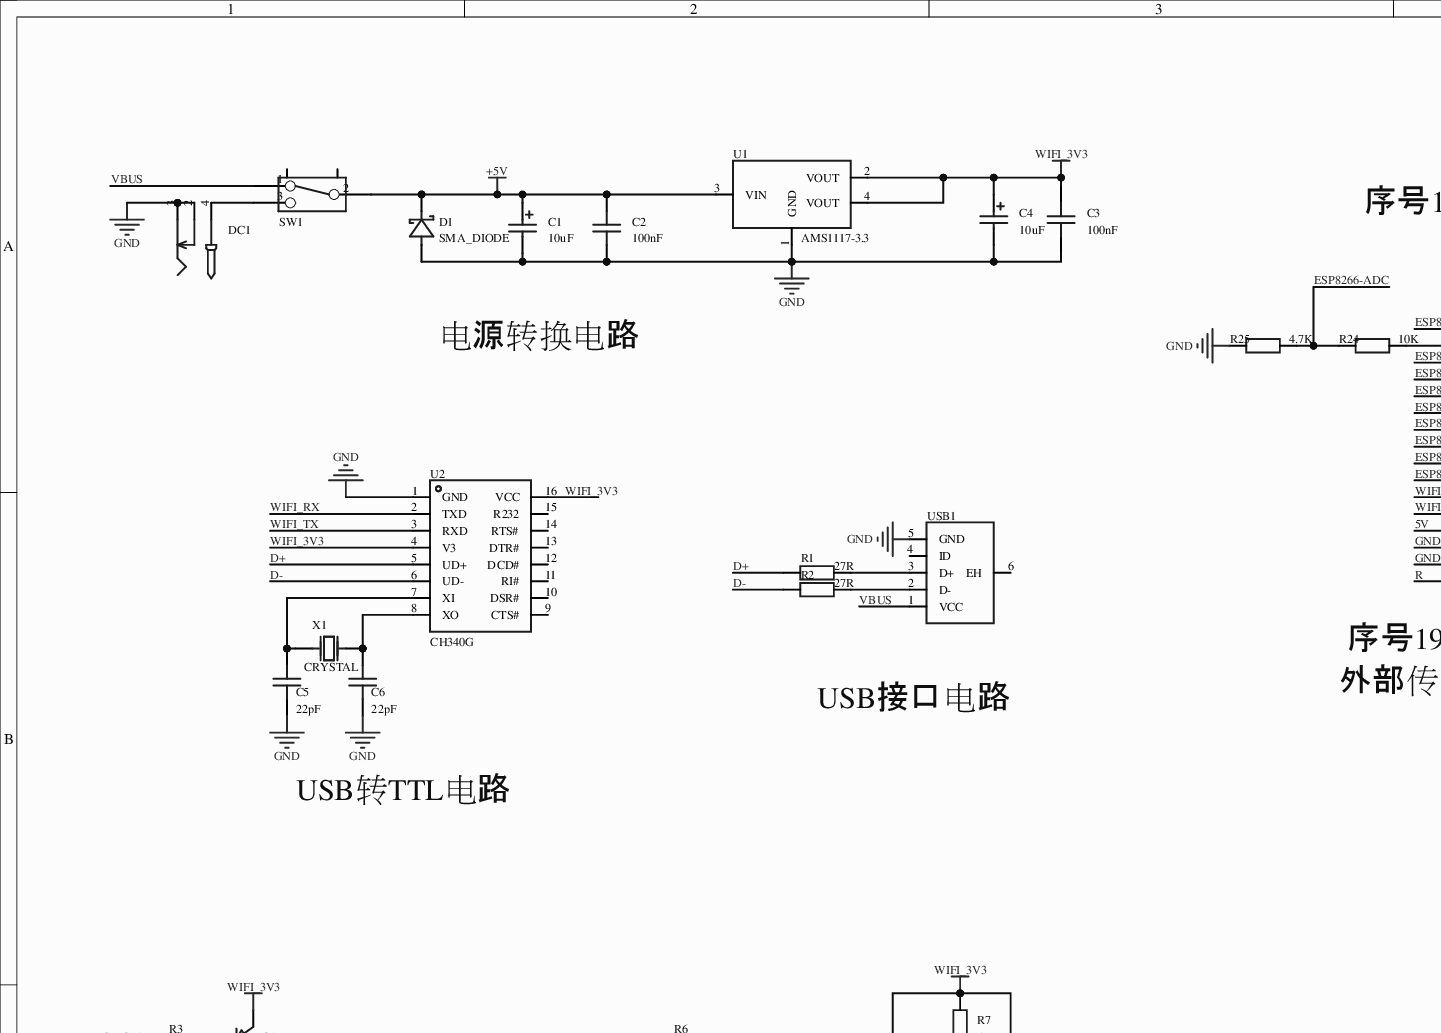
[diagram p0: MISC51905-3.schdoc, top left]
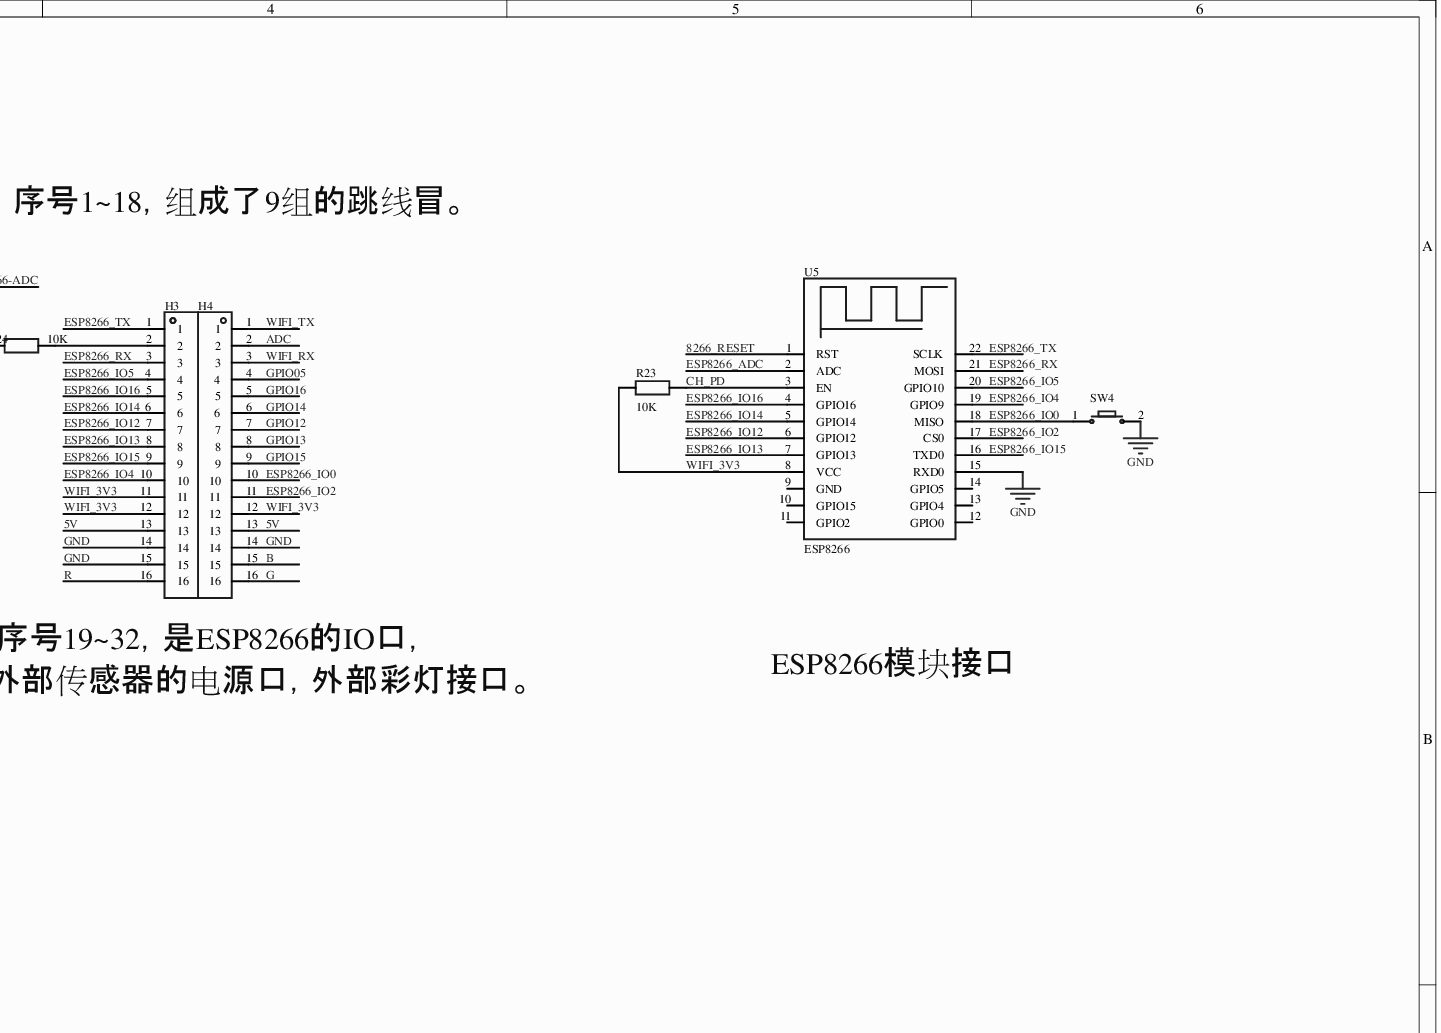
[diagram p1: MISC51905-3.schdoc, top right]
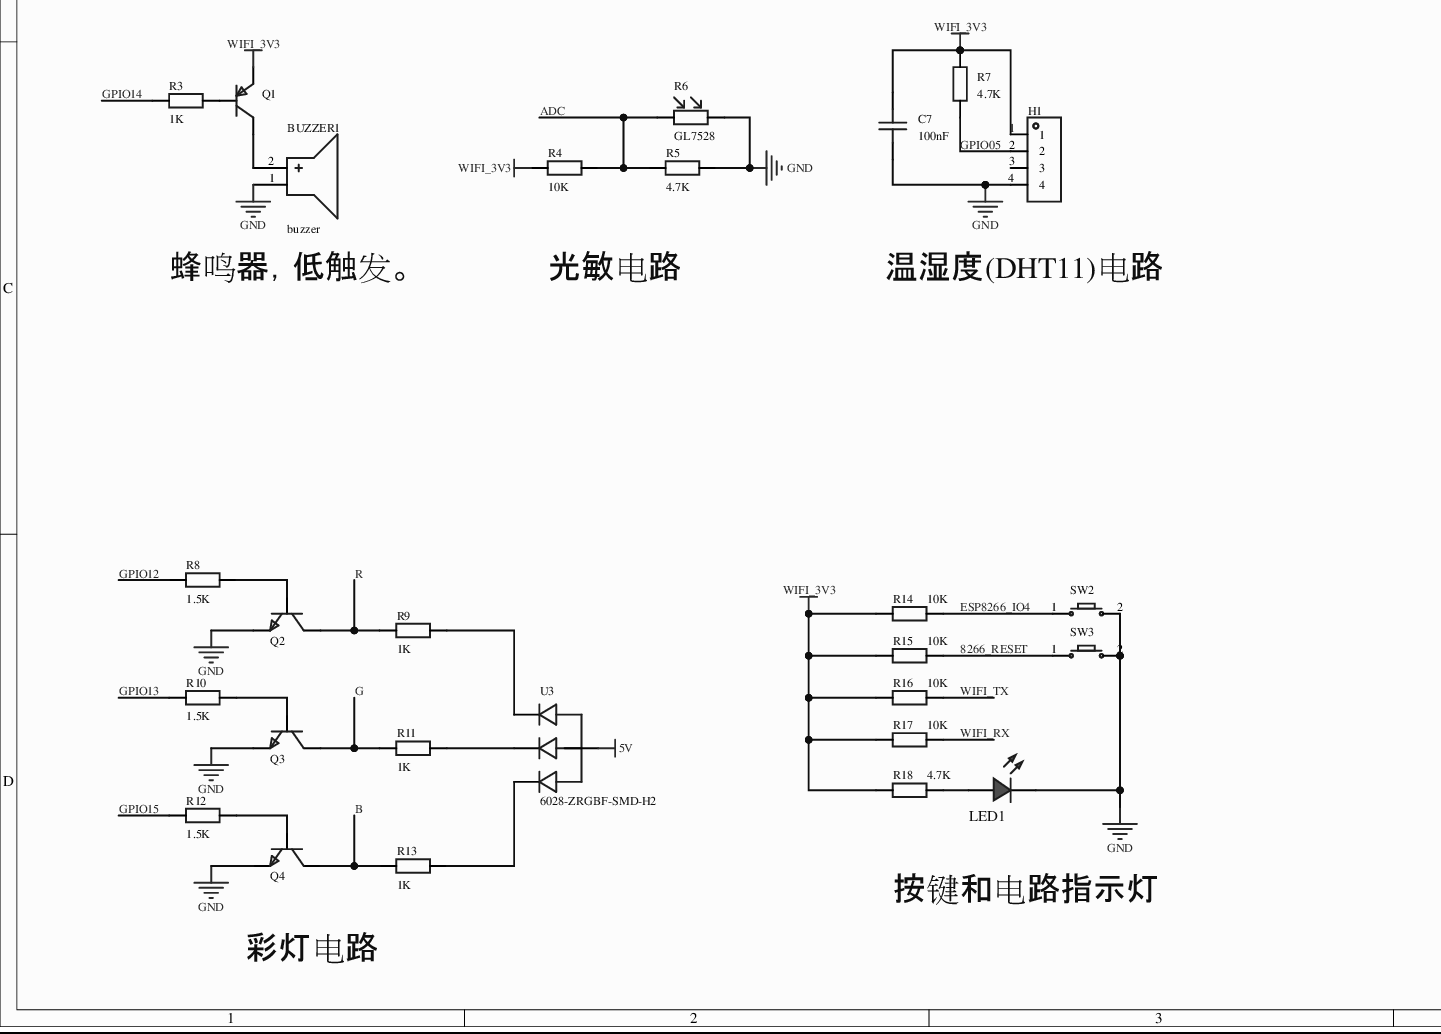
[diagram p2: MISC51905-3.schdoc, bottom left]
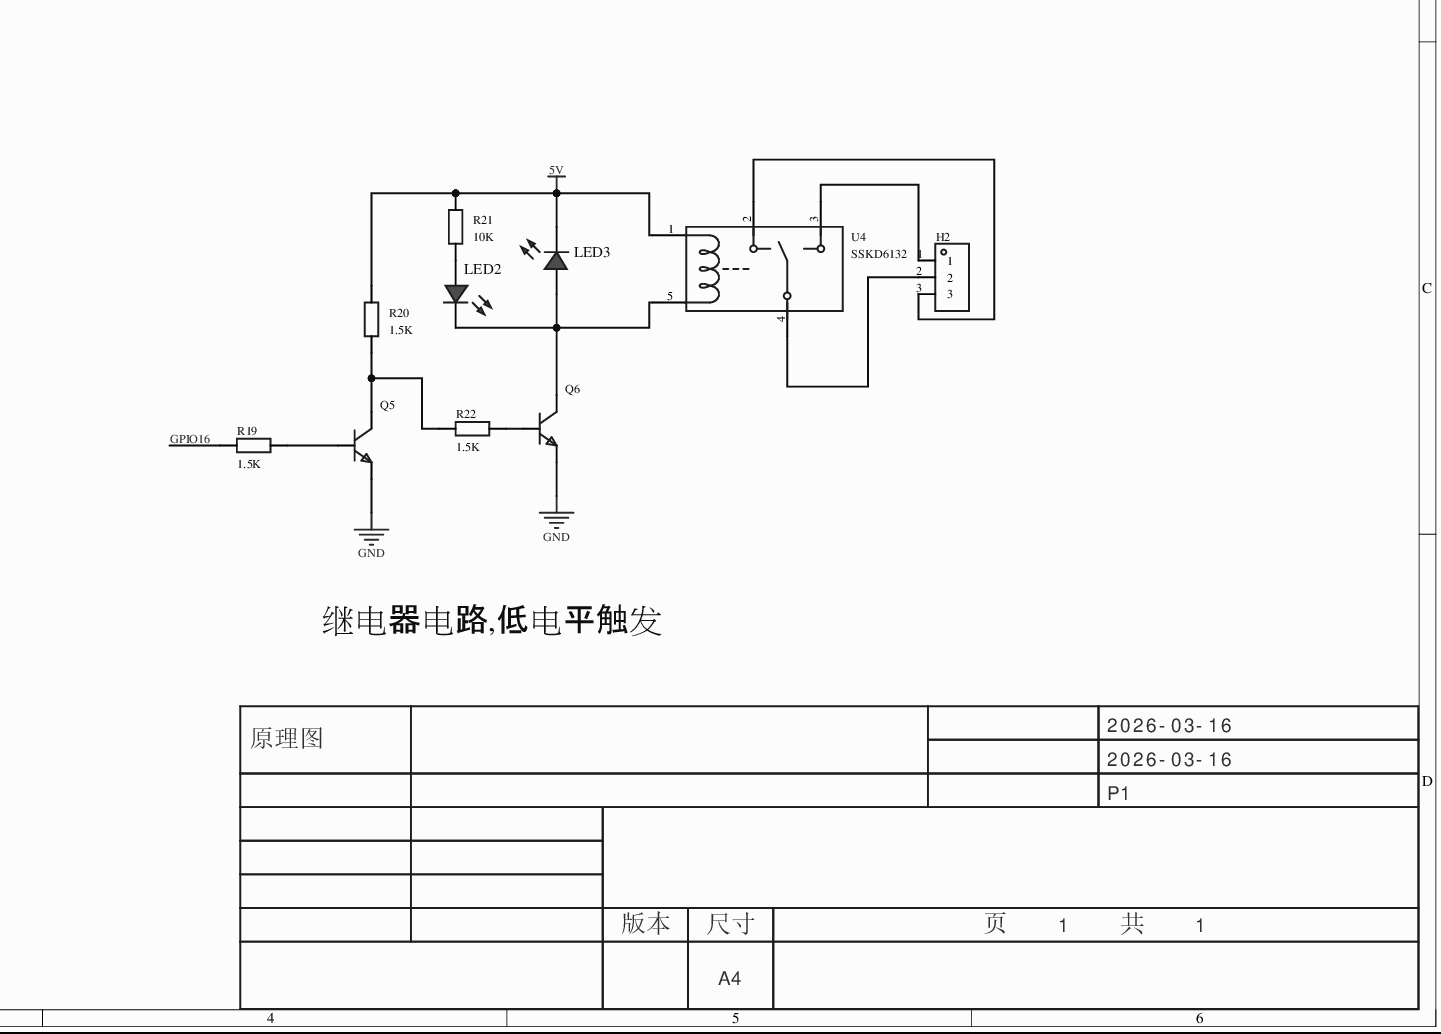
[diagram p3: MISC51905-3.schdoc, bottom right]
# Altium project MISC51905-2.PrjPcb
1 sheet, 59 parts. Net scope: global (net labels, ports and power ports of the same name join across sheets).
Board file: MISC51905.pcbdoc

## Sheet MISC51905-3.schdoc
size 420 x 297 mm; Version: V1.0; @Project Name: MISC51905; @Update Date: 2026-03-16; @Create Date: 2026-03-16; @Board Name: MISC51905; @Create Time: 19:00:49; @Page Count: 1; @Page No: 1; @Schematic Name: MISC51905; @Update Time: 19:00:49; Size: A4

### Parts
BUZZER1  buzzer  [BUZ-TH_BD12.0-P6.00-D0.9-RD]
C1  10uF  [C_Ele_SMD_5x5.4mm]
C2  100nF  [C0603]
C3  100nF  [C0603]
C4  10uF  [C_Ele_SMD_5x5.4mm]
C5  22pF  [C0603]
C6  22pF  [C0603]
C7  100nF  [C0603]
D1  SMA_DIODE  [SOD-57_BD3.8-L4.6-P9.00-D0.8-RD]
DC1  (no value)  [DC-2.0]
H1  (no value)  [HDR-TH_4P-P2.54-V-F]
H2  (no value)  [HDR-TH_3P-P2.54-V-F]
H3  (no value)  [HDR-TH_16P-P2.54-V-F]
H4  (no value)  [HDR-TH_16P-P2.54-V-F]
LED1  (no value)  [LED_0805]
LED2  (no value)  [LED_0805]
LED3  (no value)  [LED_0805]
Q1  (no value)  [S8550P_SOT]
Q2  (no value)  [S8050_SOT-23]
Q3  (no value)  [S8050_SOT-23]
Q4  (no value)  [S8050_SOT-23]
Q5  (no value)  [S8050_SOT-23]
Q6  (no value)  [S8050_SOT-23]
R1  27R  [R0603]
R2  27R  [R0603]
R3  1K  [R0805]
R4  10K  [R0805]
R5  4.7K  [R0805]
R6  GL7528  [RES-TH_L7.0-W5.9-P5.00-D0.5]
R7  4.7K  [R0805]
R8  1.5K  [R0805]
R9  1K  [R0805]
R10  1.5K  [R0805]
R11  1K  [R0805]
R12  1.5K  [R0805]
R13  1K  [R0805]
R14  10K  [R0805]
R15  10K  [R0805]
R16  10K  [R0805]
R17  10K  [R0805]
R18  4.7K  [R0805]
R19  1.5K  [R0805]
R20  1.5K  [R0805]
R21  10K  [R0805]
R22  1.5K  [R0805]
R23  10K  [R0805]
R24  10K  [Res_1/8W]
R25  4.7K  [Res_1/8W]
SW1  (no value)  [拨动开关_侧]
SW2  (no value)  [Key_SMD_3x4x2]
SW3  (no value)  [Key_SMD_3x4x2]
SW4  (no value)  [Key_SMD_3x4x2]
U1  AMS1117-3.3  [SOT-223-3_L6.5-W3.4-P2.30-LS7.0-BR]
U2  CH340G  [SOIC-16_L9.9-W3.9-P1.27-LS6.0-BL]
U3  6028-ZRGBF-SMD-H2  [LED-SMD_4P-L3.2-W2.8_ZRGBF-SMD-H2]
U4  SSKD6132  [RELAY-TH_G2R-1]
U5  ESP8266  [WIFIM-SMD_ESP-12F-ESP8266MOD]
USB1  (no value)  [USB_Micro]
X1  CRYSTAL  [CRYSTAL-SMD_L5.0-W3.2]

### Nets
5V: H3.13 H4.13 LED3.1(C) R20.2 R21.2 U3.2(COM+) U4.1
+5V: C1.1 C2.2 D1.1(K) SW1.2 U1.3(VIN)
GND: BUZZER1.1(-) C1.2 C2.1 C3.1 C4.2 C5.1 C6.1 C7.1 D1.2(A) DC1.2 DC1.3 H1.4 H3.14 H3.15 H4.14 LED1.1(C) Q2.2 Q3.2 Q4.2 Q5.2 Q6.2 R5.2 R6.2 R25.1 SW2.2 SW3.2 SW4.2 U1.1(GND) U2.1(GND) U5.15(RXD0) USB1.5(GND)
WIFI_3V3: C3.2 C4.1 C7.2 H1.1 H3.11 H3.12 H4.12 Q1.2(E) R4.1 R7.2 R14.1 R15.1 R16.1 R17.1 R18.1 R23.1 U1.2(VOUT) U1.4(VOUT) U2.4(V3) U2.16(VCC) U5.8(VCC)
8266_RESET: R15.2 SW3.1 U5.1(RST)
ADC: H4.2 R4.2 R5.1 R6.1
B: H4.15 Q4.3 R13.1
CH_PD: R23.2 U5.3(EN)
D+: R1.1 U2.5(UD+)
D-: R2.1 U2.6(UD-)
ESP8266-ADC: R24.1 R25.2
ESP8266_ADC: U5.2(ADC)
ESP8266_IO0: H4.10 SW4.1 U5.18(MISO)
ESP8266_IO2: H4.11 U5.17(CS0)
ESP8266_IO4: H3.10 R14.2 SW2.1 U5.19(GPIO9)
ESP8266_IO5: H3.4 U5.20(GPIO10)
ESP8266_IO12: H3.7 U5.6(GPIO12)
ESP8266_IO13: H3.8 U5.7(GPIO13)
ESP8266_IO14: H3.6 U5.5(GPIO14)
ESP8266_IO15: H3.9 U5.16(TXD0)
ESP8266_IO16: H3.5 U5.4(GPIO16)
ESP8266_RX: H3.3 U5.21(MOSI)
ESP8266_TX: H3.1 U5.22(SCLK)
G: H4.16 Q3.3 R11.1
GPIO05: H1.2 H4.4 R7.1
GPIO12: H4.7 R8.1
GPIO13: H4.8 R10.1
GPIO14: H4.6 R3.1
GPIO15: H4.9 R12.1
GPIO16: H4.5 R19.1
R: H3.16 Q2.3 R9.1
VBUS: SW1.1 USB1.1(VCC)
WIFI_RX: H4.3 R17.2 U2.2(TXD)
WIFI_TX: H4.1 R16.2 U2.3(RXD)
NetBUZZER1_2: BUZZER1.2(+) Q1.3(C)
NetC5_2: C5.2 U2.7(XI) X1.1(OSC1)
NetC6_2: C6.2 U2.8(XO) X1.2(OSC2)
NetDC1_4: DC1.4 SW1.3
NetH2_1: H2.1 U4.3
NetH2_2: H2.2 U4.4
NetH2_3: H2.3 U4.2
NetH3_2: H3.2 R24.2
NetLED1_2: LED1.2(A) R18.2
NetLED2_1: LED2.1(C) LED3.2(A) Q6.3 U4.5
NetLED2_2: LED2.2(A) R21.1
NetQ1_1: Q1.1(B) R3.2
NetQ2_1: Q2.1 R8.2
NetQ3_1: Q3.1 R10.2
NetQ4_1: Q4.1 R12.2
NetQ5_1: Q5.1 R19.2
NetQ5_3: Q5.3 R20.1 R22.1
NetQ6_1: Q6.1 R22.2
NetR1_2: R1.2 USB1.3(D+)
NetR2_2: R2.2 USB1.2(D-)
NetR9_2: R9.2 U3.1(R)
NetR11_2: R11.2 U3.4(B)
NetR13_2: R13.2 U3.3(G)

Not connected (* = marked no-connect by the designer): H1 3; SW1 4 5; U2 9(CTS#) 10(DSR#) 11(RI#) 12(DCD#) 13(DTR#) 14(RTS#) 15(R232); U5 9(GND) 10(GPIO15) 11(GPIO2) 12(GPIO0) 13(GPIO4) 14(GPIO5); USB1 4(ID) 6(EH)

### Notes on the sheet
- 序号1~18，组成了9组的跳线冒。
- 电源转换电路
- 序号19~32，是ESP8266的IO口，
- USB接口电路
- 外部传感器的电源口，外部彩灯接口。
- ESP8266模块接口
- USB转TTL电路
- 蜂鸣器，低触发。
- 光敏电路
- 温湿度(DHT11)电路
- 继电器电路,低电平触发
- 彩灯电路
- 按键和电路指示灯
- 2026-03-16
- 原理图
- P1
- 版本
- 尺寸
- A4
- 页    1    共    1

### Library data of the parts
BUZZER1 = buzzer: AddInBom: yes; ModelId: af17e4151ed84fc2a628230bf23763630819f05c4eef4c71ace90d822a990e87; ModelTransform: 472.44,472.176,0,270,0,0,0,0,-196.85; Symbol: BUZZER; Device: buzzer; LCSC Part Name: buzzer; SupplierPart: C9900014030; ManufacturerPart: buzzer; Supplier Footprint: buzzer; JLCPCB Part Class: Extended Part; Supplier: LCSC; ConvertToPcb: yes; FootprintName: BUZ-TH_BD12.0-P6.00-D0.9-RD; ModelName: BUZ-TH_BD12.0-P6.00-D0.9-RD
C1 C4 = C_Ele_SMD_5x5.4mm: Symbol: CAP; AddInBom: yes; Device: C_Ele_SMD_5x5.4mm; Supplier Footprint: SMD,5x5.4mm; ConvertToPcb: yes; FootprintName: C_Ele_SMD_5x5.4mm; Value: 10uF
C2 C3 C5-C7 = CAP_0603: Symbol: Capacitance; ConvertToPcb: yes; ModelId: ac125912035d415993ca9572d50418b10819f05c4eef4c71ace90d822a990e87; ModelName: C0603_L1.6-W0.8-H0.8; ModelTransform: 62.992,31.496,0,0,0,0,0,0,0; Device: CAP_0603; AddInBom: yes; Supplier Footprint: 0603; FootprintName: C0603
  C2 C3 C7: Value: 100nF
  C5 C6: Value: 22pF
D1 = SMA_DIODE: AddInBom: yes; ModelId: 9d3120876592498385ffc7c85c6b53e30819f05c4eef4c71ace90d822a990e87; ModelTransform: 354.33,149.70372,0,0,0,0,0,0,-137.795; Symbol: SMA_DIODE; Device: SMA_DIODE; LCSC Part Name: SMA_DIODE; SupplierPart: C9900013997; ManufacturerPart: SMA_DIODE; Supplier Footprint: 1N4007_SMADIODE; JLCPCB Part Class: Extended Part; Supplier: LCSC; ConvertToPcb: yes; FootprintName: SOD-57_BD3.8-L4.6-P9.00-D0.8-RD; ModelName: SOD-57_BD3.8-L4.6-P9.00-D0.8-RD
DC1 = DC-005_2.0: Symbol: DC电源接口; ConvertToPcb: yes; ModelId: f5f20b8a2308479b936ba3c2698865bb0819f05c4eef4c71ace90d822a990e87; ModelName: DC-IN-TH_DC-5520-1; ModelTransform: 372.05,551.18,582.68,90,0,0,137.8,0,-149.61; Device: DC-005_2.0; AddInBom: yes; Supplier Footprint: 插件; FootprintName: DC-2.0
H1 = HDR-F_2.54_1x4P: Symbol: 2.54-1*4P母; ConvertToPcb: yes; ModelId: d187812051054f85879fcaa51a310d8e0819f05c4eef4c71ace90d822a990e87; ModelTransform: 419.6842,98.464,0,0,0,0,0,0,-118.11; Device: HDR-F_2.54_1x4P; AddInBom: yes; SupplierPart: C2718488; Supplier Footprint: 插件; FootprintName: HDR-TH_4P-P2.54-V-F; ModelName: HDR-TH_4P-P2.54-V-F
H2 = HDR-F_2.54_1x3P: Symbol: PM254V-11-03-H85; ConvertToPcb: yes; ModelId: f3b3cc5aae9641bf9e56fc160cef875b0819f05c4eef4c71ace90d822a990e87; ModelName: HDR2.54-F-LI-1X3P; ModelTransform: 299.9994,100,0,0,0,0,0,0,-118.11; Device: HDR-F_2.54_1x3P; AddInBom: yes; SupplierPart: C541850; Supplier Footprint: 插件; FootprintName: HDR-TH_3P-P2.54-V-F
H3 H4 = HDR-F_2.54_1x16P: ConvertToPcb: yes; ModelId: 131891db3d2f4da4a154b1903ad8586e0819f05c4eef4c71ace90d822a990e87; ModelName: HDR-TH_16P-P2.54-F-LI-1X16P; ModelTransform: 1599.997,100,0,0,0,0,0,0,-118.11; Symbol: HDR-F_2.54_1x16P; Device: HDR-F_2.54_1x16P; AddInBom: yes; SupplierPart: C124409; Supplier Footprint: 插件; FootprintName: HDR-TH_16P-P2.54-V-F
LED1-LED3 = LED_0805-R: Symbol: LED_R; Convert to PCB: yes; 3D Model: 33fb9fca58e84f37a403ebeef4c28b770819f05c4eef4c71ace90d822a990e87; 3D Model Transform: 78.7,49.1,39.3,0,0,0,0,0,0; ModelName: LED-0805_R; Device: LED_0805-R; Add into BOM: yes; Supplier Footprint: 0805; FootprintName: LED_0805
Q1 = S8550_SOT_PNP: Symbol: PNP; ConvertToPcb: yes; ModelId: 9c0df02d6f3e44e889da37f3e5bf54960819f05c4eef4c71ace90d822a990e87; ModelName: SOT-23-3_L2.9-W1.4-P1.90-LS2.5-BR; ModelTransform: 98.43,114.17,37.91,0,0,0,0,0,0; Device: S8550_SOT_PNP; AddInBom: yes; Supplier Footprint: SOT-23; FootprintName: S8550P_SOT
Q2-Q6 = S8050_SOT_NPN: Symbol: NPN; ConvertToPcb: yes; ModelId: c62791f0466c4ae2a892c056b845b0ca0819f05c4eef4c71ace90d822a990e87; ModelName: SOT-23-3P_L2.9-W1.3-H1.0-LS2.4-P0.95; ModelTransform: 98.6,114.12,41.29,180,0,0,0,0,-3; Device: S8050_SOT_NPN; AddInBom: yes; Supplier Footprint: SOT-23; FootprintName: S8050_SOT-23
R1 R2 = Res_0603: Symbol: 电阻; 3D Model: fc143cca1e79419f9cd78b61e9279f080819f05c4eef4c71ace90d822a990e87; 3D Model Transform: 31.8897,63.7794,0,90,0,0,0,0,0; ConvertToPcb: yes; Device: Res_0603; Supplier Footprint: 0603; Value: 27R; AddInBom: yes; FootprintName: R0603; ModelName: R0603
R3-R5 R7 R8 R10 R12 R14-R23 = Res_0805: Symbol: 电阻; ConvertToPcb: yes; ModelId: 37a81e68749a4138bd2dfa6897b24b850819f05c4eef4c71ace90d822a990e87; ModelName: R0805_L2.0-W1.3-H0.6; ModelTransform: 78.74,51.181,0,0,0,0,0,-0.0005,0; Device: Res_0805; AddInBom: yes; Supplier Footprint: 0805; FootprintName: R0805
  R3: Value: 1K
  R4 R14-R17 R21 R23: Value: 10K
  R5 R7 R18: Value: 4.7K
  R8 R10 R12 R19 R20 R22: Value: 1.5K
R6 = GL7528: 暗电阻:-;光谱峰值(波长):-;; Manufacturer: JCHL(晶创和立); AddInBom: yes; ModelId: 7eb29834bbac436692667ec3c48270fe0819f05c4eef4c71ace90d822a990e87; ModelName: RES-TH_L7.0-W5.9-H2.5-P5.00-D0.5; ModelTransform: 232.283,275.59,0,0,0,0,0,0.005,-196.85; Symbol: GL7528; Device: GL7528; LCSC Part Name: 光敏电阻; SupplierPart: C559382; ManufacturerPart: GL7528; Supplier Footprint: 插件,P=5mm; JLCPCB Part Class: Extended Part; Datasheet: https://item.szlcsc.com/datasheet/GL7528/583274.html; Supplier: LCSC; ConvertToPcb: yes; FootprintName: RES-TH_L7.0-W5.9-P5.00-D0.5; Dark Resistance: -; Voltage - Max: -; Wavelength - Peak: -; Rise Time: -; Fall Time: -; Operating Temperature: -
R9 R11 R13 = Res_0805: Symbol: 电阻; 3D Model: 37a81e68749a4138bd2dfa6897b24b850819f05c4eef4c71ace90d822a990e87; 3D Model Transform: 78.74,51.181,0,0,0,0,0,-0.0005,0; ConvertToPcb: yes; ModelName: R0805_L2.0-W1.3-H0.6; Device: Res_0805; Value: 1K; Supplier Footprint: 0805; AddInBom: yes; FootprintName: R0805
R24 R25 = Res_AXIAL-1/8W: Symbol: 电阻; 3D Model: b2b5ae7ae4c642178fe0039925c86a3f0819f05c4eef4c71ace90d822a990e87; 3D Model Transform: 282.86,66.88,253.09,0,0,0,0,0,-191; ConvertToPcb: yes; ModelName: RES-TH_BD1.8-L3.2-P7.20-D0.4; Device: Res_AXIAL-1/8W; Supplier Footprint: 轴向引线; AddInBom: yes; FootprintName: Res_1/8W
  R24: Value: 10K
  R25: Value: 4.7K
SW1 = 拨动开关_侧: Symbol: 拨动开关; 3D Model: 10ea2cc5ba004a75b38812aadef1031f0819f05c4eef4c71ace90d822a990e87; 3D Model Transform: 337.98,287.46,295.24,0,0,0,0,-57,-110; ConvertToPcb: yes; ModelName: SW-TH_SK-12D07-VG3; Device: 拨动开关_侧; Supplier Footprint: 插件; AddInBom: yes; FootprintName: 拨动开关_侧
SW2-SW4 = Key_SMD_3x4x2: Symbol: 轻触按键x2; ConvertToPcb: yes; ModelId: 63599cce708d48afbce1b0db003544770819f05c4eef4c71ace90d822a990e87; ModelName: SW-SMD_L4.0-W2.9-H2-LS5.0; ModelTransform: 196.85,114.17,79.13,0,0,0,0,0,0; Device: Key_SMD_3x4x2; AddInBom: yes; Supplier Footprint: SMD; FootprintName: Key_SMD_3x4x2
U1 = AMS1117-3.3_C6186: 输出类型:固定;工作电压:16V;输出电压:3.3V;输出电流:1A;电源纹波抑制比(PSRR):72dB@(120Hz);输出极性:正极;; Manufacturer: AMS; AddInBom: yes; ModelId: 925194bf9823436183a3e0b978a8d0760819f05c4eef4c71ace90d822a990e87; ModelName: SOT-223-4P_L6.5-W3.5-H1.6-LS7.0-P2.30; ModelTransform: 279.89794,255.905,0,180,0,0,-3.9385,-0.0005,0; Output Type: 固定; Voltage - Supply: 16V; Output Voltage: 3.3V; Output Current: 1A; Voltage Dropout: 1.1V@(800mA); standby current: 5mA; Noise: 0.003%Vout; Output Configuration: 正极; Number of Outputs: 1; Symbol: AMS1117-3.3; Device: AMS1117-3.3_C6186; LCSC Part Name: 输出3.3V 1A; SupplierPart: C6186; ManufacturerPart: AMS1117-3.3; Supplier Footprint: SOT-223; JLCPCB Part Class: Basic Part; Datasheet: https://item.szlcsc.com/datasheet/AMS1117-3.3/6652.html; Supplier: LCSC; ConvertToPcb: yes; FootprintName: SOT-223-3_L6.5-W3.4-P2.30-LS7.0-BR; Power Supply Rejection Ratio (PSRR): 72dB@(120Hz); Features: 过流保护；过热保护; Operating Temperature: -40℃~+125℃
U2 = CH340G: 应用功能:USB转UART;接口协议:USB 2.0;数据速率:2Mbps;; Manufacturer: WCH(南京沁恒); AddInBom: yes; ModelId: c21ec766ec2643efb3352f8441994f4e0819f05c4eef4c71ace90d822a990e87; ModelName: SOIC-16_L9.9-W3.9-H1.8-LS6.0-P1.27; ModelTransform: 389.763,236.454,0,0,0,0,0,0,0; Protocol: USB 2.0; Supply Voltage: 5V；3.3V; Data Rate: 2Mbps; Symbol: CH340G; Device: CH340G; LCSC Part Name: USB转串口芯片CH340; SupplierPart: C14267; ManufacturerPart: CH340G; Supplier Footprint: SOP-16; JLCPCB Part Class: Extended Part; Datasheet: https://atta.szlcsc.com/upload/public/pdf/source/20240313/8510303D24D987FBF1AD30058571F10E.pdf; Supplier: LCSC; ConvertToPcb: yes; FootprintName: SOIC-16_L9.9-W3.9-P1.27-LS6.0-BL; Applications Function: USB转UART; Operating Temperature: -40℃~+85℃
U3 = 6028-ZRGBF-SMD-H2: AddInBom: yes; ModelId: 24ff06aa4fd343b386150bae5c3ec47f0819f05c4eef4c71ace90d822a990e87; ModelTransform: 236.22,110.63,0,180,0,0,0,0,-35.433; Symbol: 6028-ZRGBF-SMD-H2; Device: 6028-ZRGBF-SMD-H2; LCSC Part Name: 6028-ZRGBF-SMD-H2; SupplierPart: C9900095081; ManufacturerPart: 6028-ZRGBF-SMD-H2; Supplier Footprint: SMD-LED-6028-ZRGBF-SMD-H2; JLCPCB Part Class: Extended Part; Supplier: LCSC; ConvertToPcb: yes; FootprintName: LED-SMD_4P-L3.2-W2.8_ZRGBF-SMD-H2; ModelName: LED-SMD_4P-L3.2-W2.8_ZRGBF-SMD-H2
U4 = SSKD6132: AddInBom: yes; ModelId: fe99462dd15043c98af5adb0e5338dda0819f05c4eef4c71ace90d822a990e87; ModelTransform: 1141.73,511.81,0,0,0,0,26.417,-0.354,-157.48; Symbol: SSKD6132; Device: SSKD6132; LCSC Part Name: SSKD6132; SupplierPart: C9900012103; ManufacturerPart: SSKD6132; Supplier Footprint: RELAY-TH_G2R-1; JLCPCB Part Class: Extended Part; Supplier: LCSC; ConvertToPcb: yes; FootprintName: RELAY-TH_G2R-1; ModelName: RELAY-TH_G2R-1
U5 = ESP8266: AddInBom: yes; ModelId: c53b8c57aa74447bb5071c1a48f7c2190819f05c4eef4c71ace90d822a990e87; ModelName: WIFIM-SMD_WIFI-L24.0-W16.0-H3.1; ModelTransform: 630.707,945.274,0,90,0,0,-162.403,0,0; Symbol: ESP8266; Device: ESP8266; LCSC Part Name: ESP8266; SupplierPart: C9900003049; ManufacturerPart: ESP8266; Supplier Footprint: WIFIM-SMD; JLCPCB Part Class: Extended Part; Supplier: LCSC; ConvertToPcb: yes; FootprintName: WIFIM-SMD_ESP-12F-ESP8266MOD
USB1 = USB_Micro-B: AddInBom: yes; ModelId: 4933c3c2baea4358bc2662474c6970960819f05c4eef4c71ace90d822a990e87; ModelName: MINI-USB-SMD_MICRO-4P-DIP; ModelTransform: 295.275,240.157,0,180,0,0,0,-34.253,-39.37; Symbol: USB_Micro; Device: USB_Micro-B; ConvertToPcb: yes; FootprintName: USB_Micro; Supplier Footprint: SMD
X1 = X50328MSB2GI: 晶振类型:贴片晶振;频率:8MHz;常温频差:±10ppm;负载电容:20pF;频率稳定度:±20ppm;; Manufacturer: YXC(扬兴晶振); AddInBom: yes; ModelId: d7c39c66443246ff83c2003c1e1eb6f10819f05c4eef4c71ace90d822a990e87; ModelTransform: 196.85,125.984,0,0,0,0,0,0,0; Normal temperature Frequency Tolerance: ±10ppm; Load Capacitance: 20pF; Frequency Stability: ±20ppm; Symbol: X50328MSB2GI; Device: X50328MSB2GI; Value: CRYSTAL; LCSC Part Name: YSX530GA 8MHZ 2P 5032 20PF ±10PPM -40~85℃ (±20PPM); ManufacturerPart: X50328MSB2GI; Supplier Footprint: SMD5032-2P; JLCPCB Part Class: Basic Part; Datasheet: https://item.szlcsc.com/datasheet/X50328MSB2GI/117214.html; Supplier: LCSC; ConvertToPcb: yes; FootprintName: CRYSTAL-SMD_L5.0-W3.2; ModelName: CRYSTAL-SMD_L5.0-W3.2; Type: 贴片晶振; Operating Temperature: -40℃~+85℃